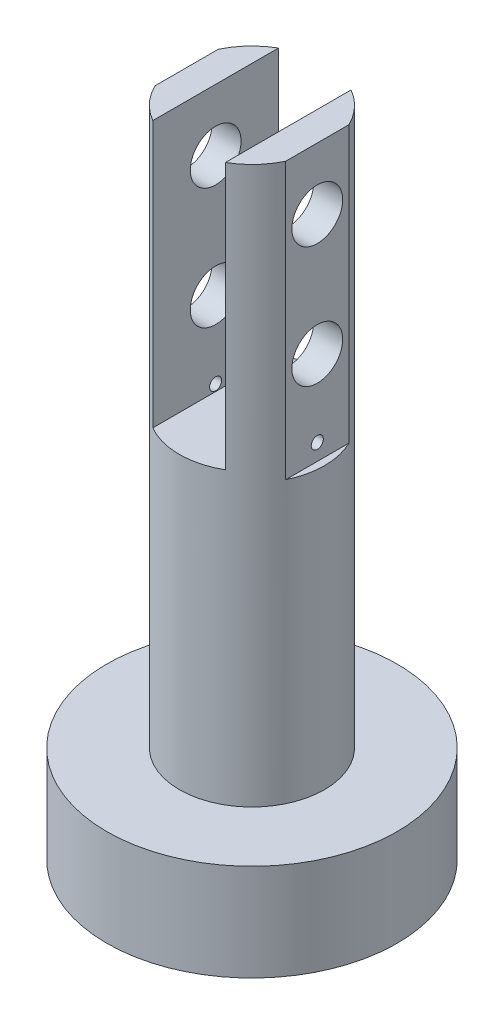
from build123d import *

# Parameters (mm, degrees)
SKETCH_1_R                = 30
EXTRUDE_1_DEPTH           = 20
SKETCH_2_R                = 15
EXTRUDE_2_DEPTH           = 115
SKETCH_3_W                = 15
SKETCH_3_H                = 65.275195259
CUT_EXTRUDE_1_DEPTH       = 50
SKETCH_4_W                = 11.214536165
SKETCH_4_H                = 73.146220951
CUT_EXTRUDE_2_DEPTH       = 25
HOLE_WIZARD_10_5_10_5_1_D = 10.5
HOLE_WIZARD_M3_1_D        = 2.5


with BuildPart() as part:
    # 草图1 → 凸台-拉伸1 (new body)
    with BuildSketch(Plane(origin=(0, 0, 0), x_dir=(1, 0, 0), z_dir=(0, 1, 0))):
        with Locations(Location((0, 0, 0), (0, 0, 270))):
            Circle(SKETCH_1_R)
    extrude(amount=EXTRUDE_1_DEPTH)

    # 草图2 → 凸台-拉伸2 (add)
    with BuildSketch(Plane(origin=(0, 20, 0), x_dir=(1, 0, 0), z_dir=(0, 1, 0))):
        with Locations(Location((0, 0, 0), (0, 0, 270))):
            Circle(SKETCH_2_R)
    extrude(amount=EXTRUDE_2_DEPTH)

    # 草图3 → 切除-拉伸1 (cut, symmetric)
    with BuildSketch(Plane.XY):
        with Locations((0, 112.63759763)):
            Rectangle(SKETCH_3_W, SKETCH_3_H)
    extrude(amount=CUT_EXTRUDE_1_DEPTH, both=True, mode=Mode.SUBTRACT)

    # 草图4 → 切除-拉伸2 (cut, symmetric)
    with BuildSketch(Plane.XY):
        with Locations((19.107268082, 114.573110476)):
            Rectangle(SKETCH_4_W, SKETCH_4_H)
        with Locations((-19.107268082, 114.573110476)):
            Rectangle(SKETCH_4_W, SKETCH_4_H)
    extrude(amount=CUT_EXTRUDE_2_DEPTH, both=True, mode=Mode.SUBTRACT)

    # Ø10.5 (10.5) 直径孔1 (through all)
    with Locations(Plane(origin=(13.5, 0, 0), x_dir=(0, 0, -1), z_dir=(1, 0, 0))):
        with Locations((0, 97.25), (0, 122.25)):
            Hole(HOLE_WIZARD_10_5_10_5_1_D / 2)

    # M3 螺纹孔1 (through all)
    with Locations(Plane.ZY.offset(13.5)):
        with Locations((0, 81.4)):
            Hole(HOLE_WIZARD_M3_1_D / 2)


solid = part.part
